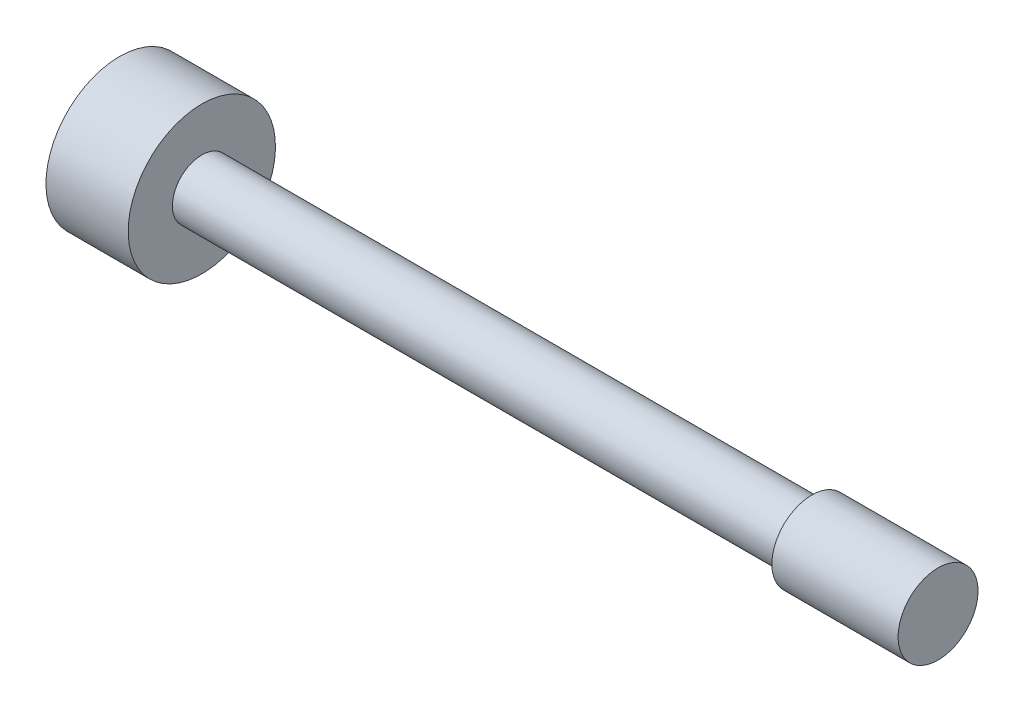
SolidWorks part; units mm, degrees
ref_plane "Front Plane" through (0, 0, 0) normal (0, 0, 1) x (1, 0, 0)
ref_plane "Top Plane" through (0, 0, 0) normal (0, 1, 0) x (1, 0, 0)
ref_plane "Right Plane" through (0, 0, 0) normal (1, 0, 0) x (0, 0, -1)
sketch "Sketch1" plane through (0, 0, 0) normal (0, 0, 1) x (1, 0, 0)
  line L0 (0, 0) -> (0, 3.5)
  line L1 (0, 3.5) -> (3.91, 3.5)
  line L2 (3.91, 3.5) -> (3.91, 1.4)
  line L3 (3.91, 1.4) -> (32.91, 1.4)
  line L5 (38.91, 0) -> (0, 0)
  line L6 (32.91, 1.4) -> (32.91, 1.9)
  line L7 (32.91, 1.9) -> (38.91, 1.9)
  line L8 (38.91, 0) -> (38.91, 1.9)
  dimension "D1" = 3.5
  dimension "D2" = 3.91
  dimension "D3" = 35
  dimension "D4" = 6
  dimension "D5" = 1.4
  dimension "D6" = 1.9
revolve "Revolve1" add sketch "Sketch1" angle 360 about L5
cosmetic thread "Cosmetic Thread1" parameters "D2"=3
